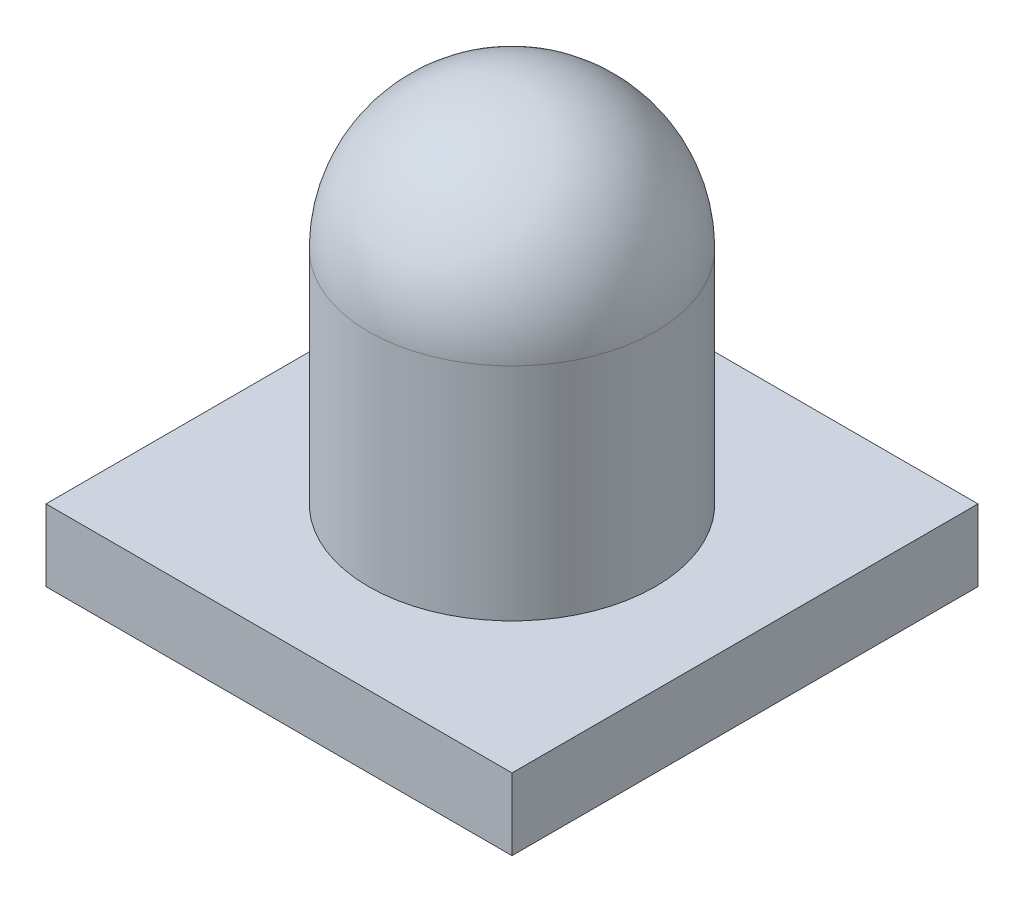
from build123d import *

# Parameters (mm, degrees)
SKETCH1_W           = 65
SKETCH1_H           = 65
BOSS_EXTRUDE1_DEPTH = 10
SKETCH2_R           = 20
BOSS_EXTRUDE2_DEPTH = 50.8
FILLET1_R           = 20
SKETCH3_R           = 1.5
CUT_EXTRUDE1_DEPTH  = 5


with BuildPart() as part:
    # Sketch1 → Boss-Extrude1 (new body)
    with BuildSketch(Plane(origin=(0, 0, 0), x_dir=(1, 0, 0), z_dir=(0, 1, 0))):
        Rectangle(SKETCH1_W, SKETCH1_H)
    extrude(amount=BOSS_EXTRUDE1_DEPTH)

    # Sketch2 → Boss-Extrude2 (add)
    with BuildSketch(Plane(origin=(0, 10, 0), x_dir=(1, 0, 0), z_dir=(0, 1, 0))):
        with Locations(Location((0, 0, 0), (0, 0, 270))):
            Circle(SKETCH2_R)
    extrude(amount=BOSS_EXTRUDE2_DEPTH)

    # Fillet1
    fillet1_edges = [part.edges().sort_by_distance(p)[0] for p in [
        (0, 60.8, -20),
    ]]
    fillet(fillet1_edges, radius=FILLET1_R)

    # Sketch3 → Cut-Extrude1 (cut)
    with BuildSketch(Plane.XZ):
        with Locations(Location((24, 18, 0), (0, 0, 270))):
            Circle(SKETCH3_R)
        with Locations(Location((-24, 18, 0), (0, 0, 270))):
            Circle(SKETCH3_R)
        with Locations(Location((-24, -18, 0), (0, 0, 270))):
            Circle(SKETCH3_R)
        with Locations(Location((24, -18, 0), (0, 0, 270))):
            Circle(SKETCH3_R)
    extrude(amount=-CUT_EXTRUDE1_DEPTH, mode=Mode.SUBTRACT)


solid = part.part
